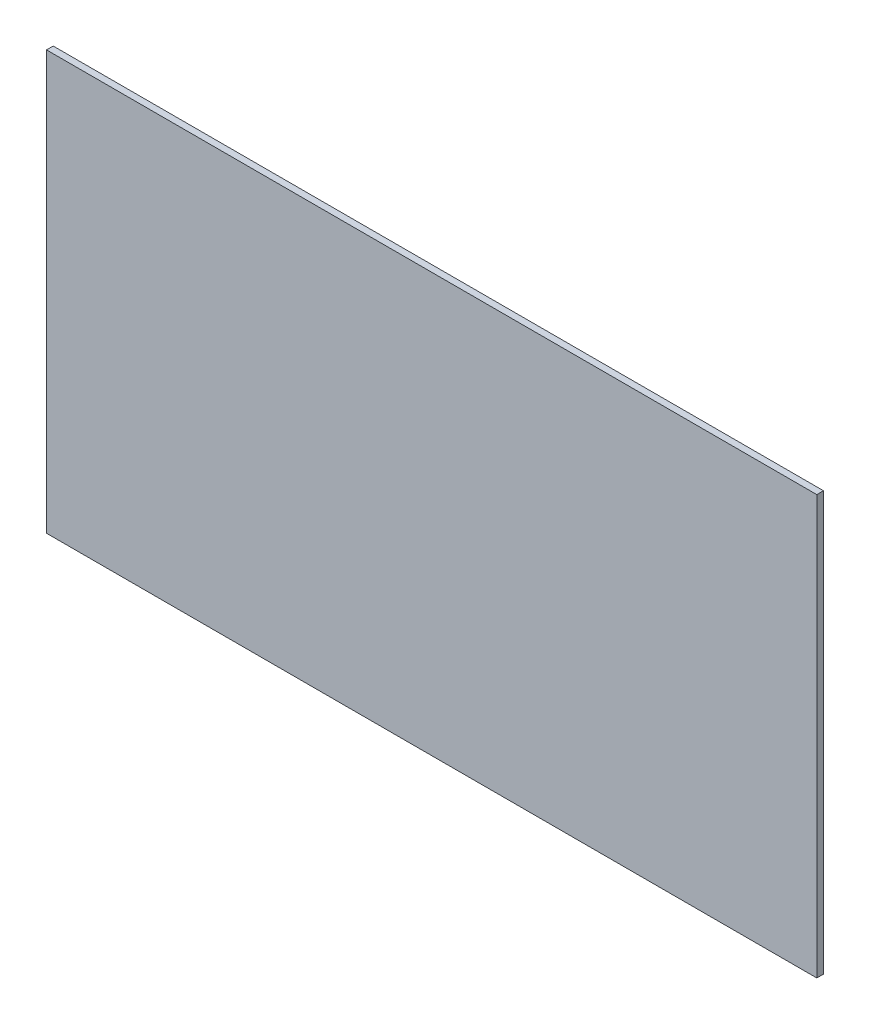
SolidWorks part; units mm, degrees
ref_plane "Front Plane" through (0, 0, 0) normal (0, 0, 1) x (1, 0, 0)
ref_plane "Top Plane" through (0, 0, 0) normal (0, 1, 0) x (1, 0, 0)
ref_plane "Right Plane" through (0, 0, 0) normal (1, 0, 0) x (0, 0, -1)
sketch "Sketch1" plane through (0, 0, 0) normal (0, 0, 1) x (1, 0, 0)
  line L1 (460, 250) -> (-460, 250)
  line L2 (460, 250) -> (460, -250)
  line L3 (460, -250) -> (-460, -250)
  line L4 (-460, 250) -> (-460, -250)
  line L5 (460, 250) -> (-460, -250) construction
  line L6 (460, -250) -> (-460, 250) construction
  point P0 (0, 0)
  dimension "D1" = 920
  dimension "D2" = 500
extrude "Boss-Extrude1" add sketch "Sketch1" along normal blind 8
